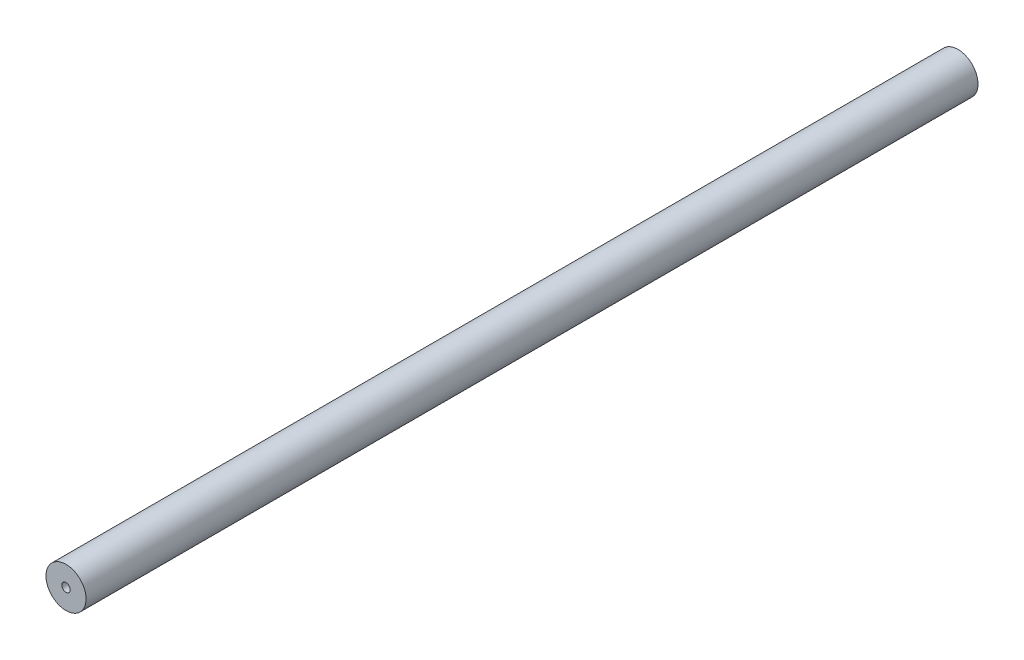
from build123d import *

# Parameters (mm, degrees)
SKETCH_1_R             = 10
EXTRUDE_1_DEPTH        = 445
HOLE_WIZARD_M5_1_D     = 4.2
HOLE_WIZARD_M5_1_DEPTH = 15
HOLE_WIZARD_M5_1_TIP   = 1.2618073
HOLE_WIZARD_M5_2_D     = 4.2
HOLE_WIZARD_M5_2_DEPTH = 15
HOLE_WIZARD_M5_2_TIP   = 1.2618073


with BuildPart() as part:
    # 草图1 → 凸台-拉伸1 (new body)
    with BuildSketch(Plane.XY):
        Circle(SKETCH_1_R)
    extrude(amount=EXTRUDE_1_DEPTH)

    # M5 螺纹孔1
    with Locations(Plane.XY.offset(445)):
        with Locations((0, 0)):
            Hole(HOLE_WIZARD_M5_1_D / 2, depth=HOLE_WIZARD_M5_1_DEPTH)
            with Locations((0, 0, -(HOLE_WIZARD_M5_1_DEPTH + HOLE_WIZARD_M5_1_TIP / 2))):  # 118° drill point
                Cone(0, HOLE_WIZARD_M5_1_D / 2, HOLE_WIZARD_M5_1_TIP, mode=Mode.SUBTRACT)

    # M5 螺纹孔2
    with Locations(Plane(origin=(0, 0, 0), x_dir=(-1, 0, 0), z_dir=(0, 0, -1))):
        with Locations((0, 0)):
            Hole(HOLE_WIZARD_M5_2_D / 2, depth=HOLE_WIZARD_M5_2_DEPTH)
            with Locations((0, 0, -(HOLE_WIZARD_M5_2_DEPTH + HOLE_WIZARD_M5_2_TIP / 2))):  # 118° drill point
                Cone(0, HOLE_WIZARD_M5_2_D / 2, HOLE_WIZARD_M5_2_TIP, mode=Mode.SUBTRACT)


solid = part.part
